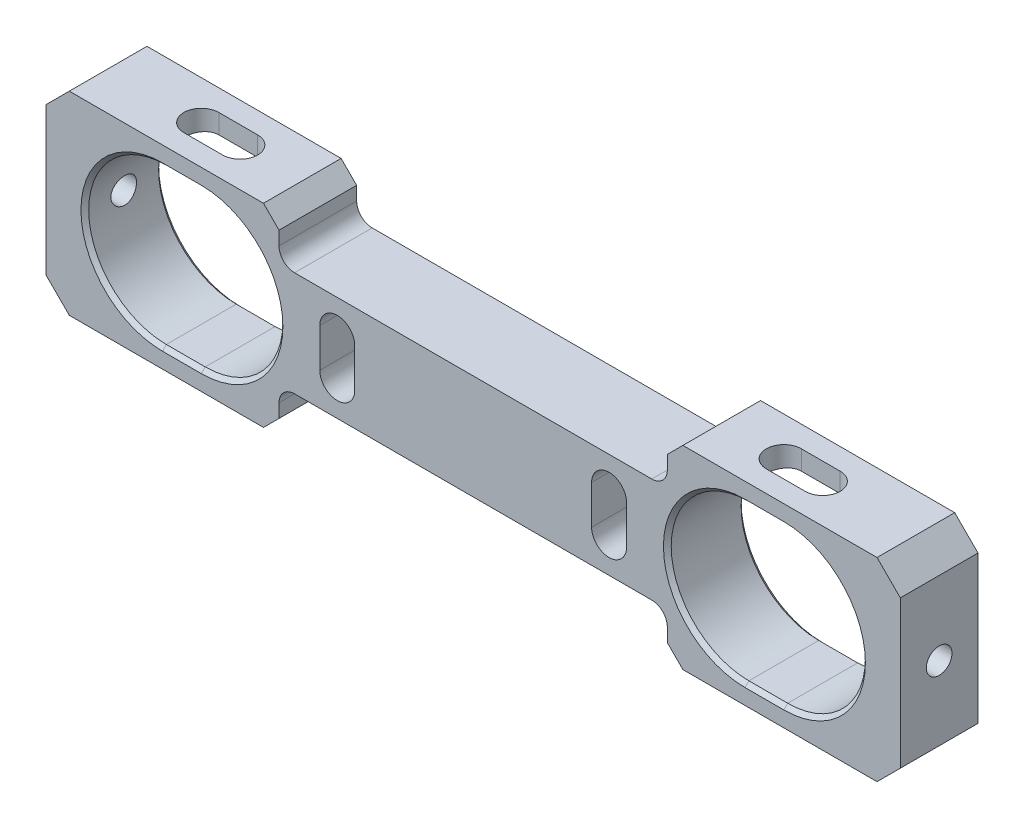
from build123d import *

# Parameters (mm, degrees)
SKETCH1_W              = 110
SKETCH1_H              = 25
BOSS_EXTRUDE1_DEPTH    = 5
CUT_EXTRUDE1_DEPTH     = 58.282196187
CHAMFER1_SIZE          = 3
CHAMFER2_SIZE          = 0.5
CUT_EXTRUDE2_DEPTH     = 58.282196187
CUT_EXTRUDE3_REACH     = 62.622
M4_TAPPED_HOLE1_REACH  = 112.821
M4_TAPPED_HOLE1_BORE_R = 1.65
M4_TAPPED_HOLE2_REACH  = 112.821
M4_TAPPED_HOLE2_BORE_R = 1.65
CUT_EXTRUDE4_DEPTH     = 4.5
SKETCH12_W             = 50
SKETCH12_H             = 5.75
CUT_EXTRUDE5_DEPTH     = 58.282196305
FILLET1_R              = 2
CHAMFER3_SIZE          = 2


with BuildPart() as part:
    # Sketch1 → Boss-Extrude1 (new, symmetric)
    with BuildSketch(Plane.XY):
        Rectangle(SKETCH1_W, SKETCH1_H)
    extrude(amount=BOSS_EXTRUDE1_DEPTH, both=True)

    # Sketch2 → Cut-Extrude1 (cut, through all)
    with BuildSketch(Plane.XY.offset(5)):
        with BuildLine():
            Line((35, 10), (40, 10))
            ThreePointArc((40, 10), (50, 0), (40, -10))
            Line((40, -10), (35, -10))
            ThreePointArc((35, -10), (25, 0), (35, 10))
        make_face()
        with BuildLine():
            Line((-40, 10), (-35, 10))
            ThreePointArc((-35, 10), (-25, 0), (-35, -10))
            Line((-35, -10), (-40, -10))
            ThreePointArc((-40, -10), (-50, 0), (-40, 10))
        make_face()
    extrude(amount=-CUT_EXTRUDE1_DEPTH, mode=Mode.SUBTRACT)

    # Chamfer1
    chamfer1_edges = [part.edges().sort_by_distance(p)[0] for p in [
        (55, -12.5, 0),
        (-55, -12.5, 0),
        (-55, 12.5, 0),
        (55, 12.5, 0),
    ]]
    chamfer(chamfer1_edges, length=CHAMFER1_SIZE)

    # Chamfer2
    chamfer2_edges = [part.edges().sort_by_distance(p)[0] for p in [
        (25, 0, -5),
        (37.5, 10, -5),
        (50, 0, -5),
        (37.5, -10, -5),
        (25, 0, 5),
        (37.5, -10, 5),
        (50, 0, 5),
        (37.5, 10, 5),
        (-50, 0, -5),
        (-37.5, 10, -5),
        (-25, 0, -5),
        (-37.5, -10, -5),
        (-50, 0, 5),
        (-37.5, -10, 5),
        (-25, 0, 5),
        (-37.5, 10, 5),
    ]]
    chamfer(chamfer2_edges, length=CHAMFER2_SIZE)

    # Sketch3 → Cut-Extrude2 (cut, through all)
    with BuildSketch(Plane.XY.offset(5)):
        with BuildLine():
            Line((19.75, 2.5), (19.75, -2.5))
            ThreePointArc((19.75, -2.5), (17.5, -4.75), (15.25, -2.5))
            Line((15.25, -2.5), (15.25, 2.5))
            ThreePointArc((15.25, 2.5), (17.5, 4.75), (19.75, 2.5))
        make_face()
        with BuildLine():
            Line((-15.25, 2.5), (-15.25, -2.5))
            ThreePointArc((-15.25, -2.5), (-17.5, -4.75), (-19.75, -2.5))
            Line((-19.75, -2.5), (-19.75, 2.5))
            ThreePointArc((-19.75, 2.5), (-17.5, 4.75), (-15.25, 2.5))
        make_face()
    extrude(amount=-CUT_EXTRUDE2_DEPTH, mode=Mode.SUBTRACT)

    # Sketch6 → Cut-Extrude3 (cut, up to next)
    with BuildSketch(Plane(origin=(0, 12.5, 0), x_dir=(1, 0, 0), z_dir=(0, 1, 0)), mode=Mode.PRIVATE) as cut_extrude3_sk1:
        with BuildLine():
            Line((-40, 2.25), (-35, 2.25))
            ThreePointArc((-35, 2.25), (-32.75, 0), (-35, -2.25))
            Line((-35, -2.25), (-40, -2.25))
            ThreePointArc((-40, -2.25), (-42.25, 0), (-40, 2.25))
        make_face()
    cut_extrude3_tool1 = extrude(cut_extrude3_sk1.sketch, amount=-CUT_EXTRUDE3_REACH, mode=Mode.PRIVATE) & part.part
    # Sketch6 → Cut-Extrude3 (cut, up to next)
    with BuildSketch(Plane(origin=(0, 12.5, 0), x_dir=(1, 0, 0), z_dir=(0, 1, 0)), mode=Mode.PRIVATE) as cut_extrude3_sk2:
        with BuildLine():
            Line((35, 2.25), (40, 2.25))
            ThreePointArc((40, 2.25), (42.25, 0), (40, -2.25))
            Line((40, -2.25), (35, -2.25))
            ThreePointArc((35, -2.25), (32.75, 0), (35, 2.25))
        make_face()
    cut_extrude3_tool2 = extrude(cut_extrude3_sk2.sketch, amount=-CUT_EXTRUDE3_REACH, mode=Mode.PRIVATE) & part.part
    add(cut_extrude3_tool1.solids().sort_by_distance((-37.5, 12.5, 0))[0], mode=Mode.SUBTRACT)
    add(cut_extrude3_tool2.solids().sort_by_distance((37.5, 12.5, 0))[0], mode=Mode.SUBTRACT)

    # M4 Tapped Hole1 bore → M4 Tapped Hole1 (cut, up to next)
    with BuildSketch(Plane(origin=(55, 0, 0), x_dir=(0, 0, -1), z_dir=(1, 0, 0)), mode=Mode.PRIVATE) as m4_tapped_hole1_sk1:
        Circle(M4_TAPPED_HOLE1_BORE_R)
    m4_tapped_hole1_tool1 = extrude(m4_tapped_hole1_sk1.sketch, amount=-M4_TAPPED_HOLE1_REACH, mode=Mode.PRIVATE) & part.part
    add(m4_tapped_hole1_tool1.solids().sort_by_distance((55, 0, 0))[0], mode=Mode.SUBTRACT)

    # M4 Tapped Hole2 bore → M4 Tapped Hole2 (cut, up to next)
    with BuildSketch(Plane.ZY.offset(55), mode=Mode.PRIVATE) as m4_tapped_hole2_sk1:
        Circle(M4_TAPPED_HOLE2_BORE_R)
    m4_tapped_hole2_tool1 = extrude(m4_tapped_hole2_sk1.sketch, amount=-M4_TAPPED_HOLE2_REACH, mode=Mode.PRIVATE) & part.part
    add(m4_tapped_hole2_tool1.solids().sort_by_distance((-55, 0, 0))[0], mode=Mode.SUBTRACT)

    # Sketch11 → Cut-Extrude4 (cut)
    with BuildSketch(Plane(origin=(0, 0, -5), x_dir=(-1, 0, 0), z_dir=(0, 0, -1))):
        with BuildLine():
            Line((-13.5, 2.5), (-13.5, -2.5))
            ThreePointArc((-13.5, -2.5), (-17.5, -6.5), (-21.5, -2.5))
            Line((-21.5, -2.5), (-21.5, 2.5))
            ThreePointArc((-21.5, 2.5), (-17.5, 6.5), (-13.5, 2.5))
        make_face()
        with BuildLine():
            Line((21.5, 2.5), (21.5, -2.5))
            ThreePointArc((21.5, -2.5), (17.5, -6.5), (13.5, -2.5))
            Line((13.5, -2.5), (13.5, 2.5))
            ThreePointArc((13.5, 2.5), (17.5, 6.5), (21.5, 2.5))
        make_face()
    extrude(amount=-CUT_EXTRUDE4_DEPTH, mode=Mode.SUBTRACT)

    # Sketch12 → Cut-Extrude5 (cut, through all)
    with BuildSketch(Plane.XY.offset(5)):
        with Locations((0, -9.625)):
            Rectangle(SKETCH12_W, SKETCH12_H)
        with Locations((0, 9.625)):
            Rectangle(SKETCH12_W, SKETCH12_H)
    extrude(amount=-CUT_EXTRUDE5_DEPTH, mode=Mode.SUBTRACT)

    # Fillet1
    fillet1_edges = [part.edges().sort_by_distance(p)[0] for p in [
        (-25, -6.75, 0),
        (25, -6.75, 0),
        (-25, 6.75, 0),
        (25, 6.75, 0),
    ]]
    fillet(fillet1_edges, radius=FILLET1_R)

    # Chamfer3
    chamfer3_edges = [part.edges().sort_by_distance(p)[0] for p in [
        (-25, -12.5, 0),
        (25, -12.5, 0),
        (-25, 12.5, 0),
        (25, 12.5, 0),
    ]]
    chamfer(chamfer3_edges, length=CHAMFER3_SIZE)


solid = part.part
